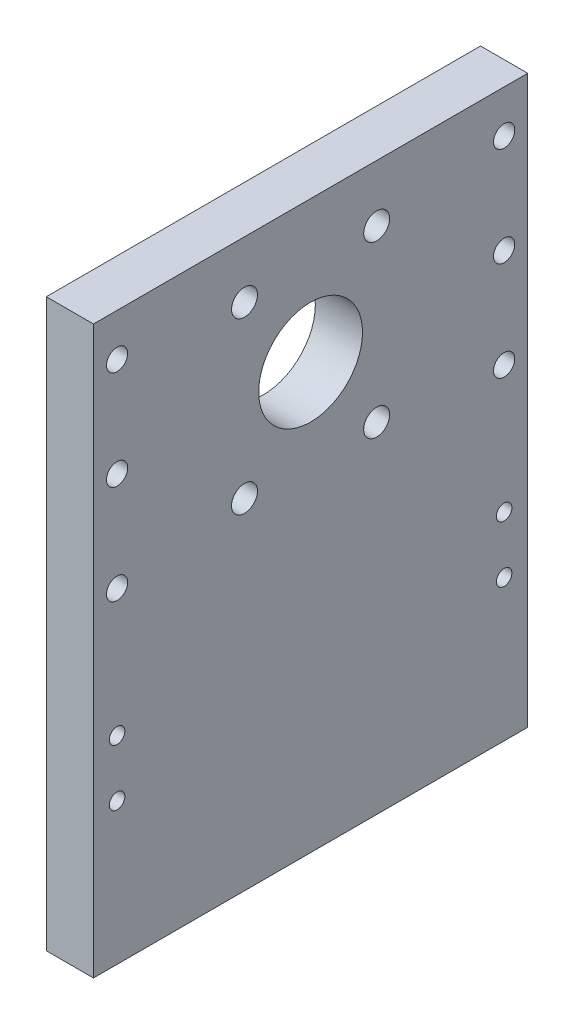
from build123d import *

# Parameters (mm, degrees)
SKETCH1_W                                           = 92
SKETCH1_H                                           = 120
BOSS_EXTRUDE1_DEPTH                                 = 5
SKETCH2_R                                           = 11
CUT_EXTRUDE1_DEPTH                                  = 77.26270386
M4_TAPPED_HOLE1_D                                   = 3.3
CBORE_FOR_M4_HEX_SOCKET_HEAD_CAP_SCREW1_D           = 4.5
CBORE_FOR_M4_HEX_SOCKET_HEAD_CAP_SCREW1_CBORE_D     = 8
CBORE_FOR_M4_HEX_SOCKET_HEAD_CAP_SCREW1_CBORE_DEPTH = 4.4
CBORE_FOR_M5_HEX_SOCKET_HEAD_CAP_SCREW1_D           = 5.5
CBORE_FOR_M5_HEX_SOCKET_HEAD_CAP_SCREW1_DEPTH       = 10.1
CBORE_FOR_M5_HEX_SOCKET_HEAD_CAP_SCREW1_CBORE_D     = 10
CBORE_FOR_M5_HEX_SOCKET_HEAD_CAP_SCREW1_CBORE_DEPTH = 5.4
CBORE_FOR_M5_HEX_SOCKET_HEAD_CAP_SCREW1_TIP         = 1.652366702


with BuildPart() as part:
    # Sketch1 → Boss-Extrude1 (new, symmetric)
    with BuildSketch(Plane(origin=(0, 0, 0), x_dir=(0, 0, -1), z_dir=(1, 0, 0))):
        Rectangle(SKETCH1_W, SKETCH1_H)
    extrude(amount=BOSS_EXTRUDE1_DEPTH, both=True)

    # Sketch2 → Cut-Extrude1 (cut, through all)
    with BuildSketch(Plane(origin=(5, 0, 0), x_dir=(0, 0, -1), z_dir=(1, 0, 0))):
        with Locations((0, 30)):
            Circle(SKETCH2_R)
    extrude(amount=-CUT_EXTRUDE1_DEPTH, mode=Mode.SUBTRACT)

    # M4 Tapped Hole1 (through all)
    with Locations(Plane(origin=(5, 0, 0), x_dir=(0, 0, -1), z_dir=(1, 0, 0))):
        with Locations((-41, -30), (-41, -18), (41, -30), (41, -18)):
            Hole(M4_TAPPED_HOLE1_D / 2)

    # CBORE for M4 Hex Socket Head Cap Screw1 (through all)
    with Locations(Plane.ZY.offset(5)):
        with Locations((-41, 51), (-41, 30), (-41, 9), (41, 51), (41, 30), (41, 9)):
            CounterBoreHole(CBORE_FOR_M4_HEX_SOCKET_HEAD_CAP_SCREW1_D / 2, CBORE_FOR_M4_HEX_SOCKET_HEAD_CAP_SCREW1_CBORE_D / 2, CBORE_FOR_M4_HEX_SOCKET_HEAD_CAP_SCREW1_CBORE_DEPTH)

    # CBORE for M5 Hex Socket Head Cap Screw1
    with Locations(Plane.ZY.offset(5)):
        with Locations((-14, 48), (14, 48), (-14, 12), (14, 12)):
            CounterBoreHole(CBORE_FOR_M5_HEX_SOCKET_HEAD_CAP_SCREW1_D / 2, CBORE_FOR_M5_HEX_SOCKET_HEAD_CAP_SCREW1_CBORE_D / 2, CBORE_FOR_M5_HEX_SOCKET_HEAD_CAP_SCREW1_CBORE_DEPTH, depth=CBORE_FOR_M5_HEX_SOCKET_HEAD_CAP_SCREW1_DEPTH)
            with Locations((0, 0, -(CBORE_FOR_M5_HEX_SOCKET_HEAD_CAP_SCREW1_DEPTH + CBORE_FOR_M5_HEX_SOCKET_HEAD_CAP_SCREW1_TIP / 2))):  # 118° drill point
                Cone(0, CBORE_FOR_M5_HEX_SOCKET_HEAD_CAP_SCREW1_D / 2, CBORE_FOR_M5_HEX_SOCKET_HEAD_CAP_SCREW1_TIP, mode=Mode.SUBTRACT)


solid = part.part
